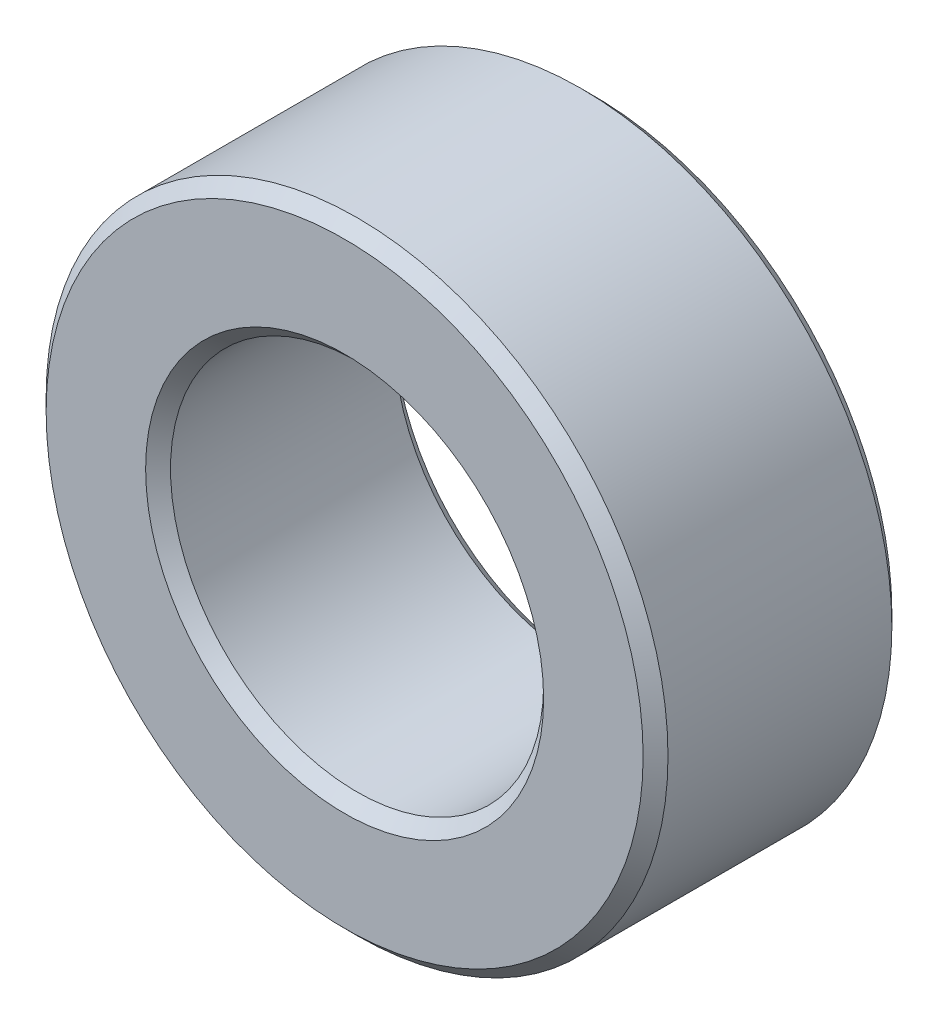
SolidWorks part; units mm, degrees
material "45#"
ref_plane "Front Plane" through (0, 0, 0) normal (0, 0, 1) x (1, 0, 0)
ref_plane "Top Plane" through (0, 0, 0) normal (0, 1, 0) x (1, 0, 0)
ref_plane "Right Plane" through (0, 0, 0) normal (1, 0, 0) x (0, 0, -1)
sketch "Sketch1" plane through (0, 0, 0) normal (0, 0, 1) x (1, 0, 0)
  circle A0 centre (0, 0) radius 25
  circle A1 centre (0, 0) radius 15
  dimension "D1" = 50
  dimension "D2" = 30
extrude "Boss-Extrude1" add sketch "Sketch1" along normal blind 20
chamfer "Chamfer1" distance 1 angle 45 4 edges at (15, 0, 0) (15, 0, 20) (25, 0, 0) (25, 0, 20)
